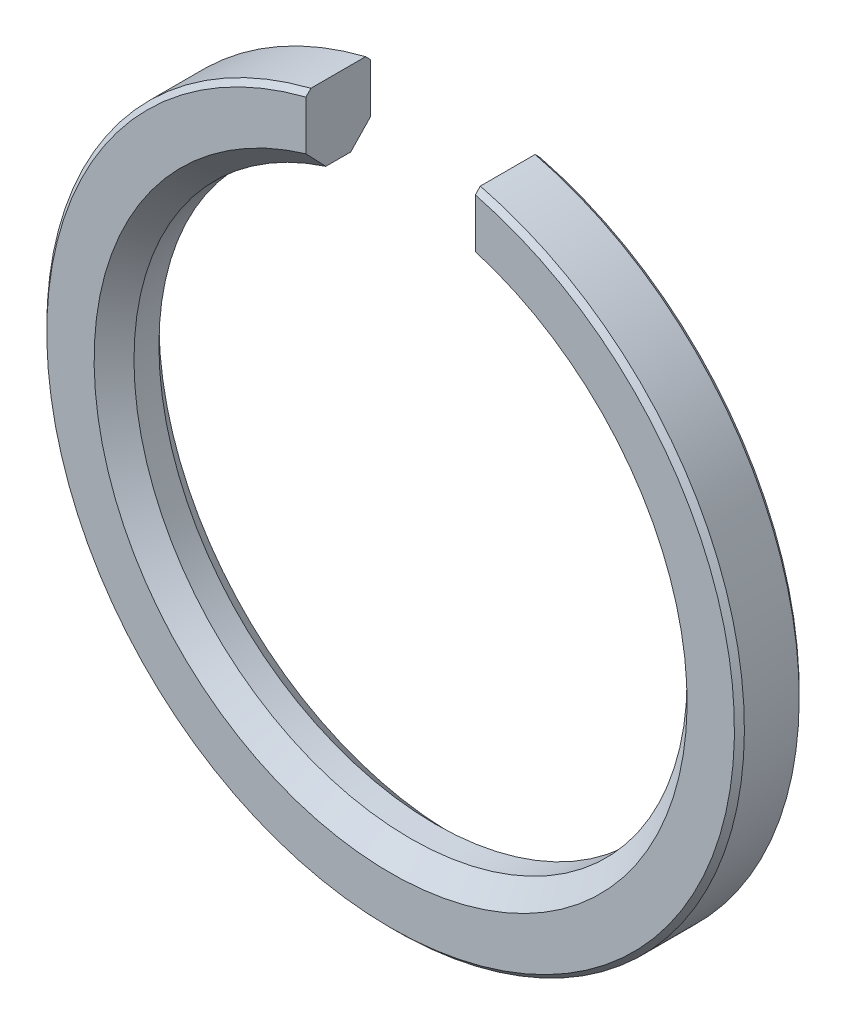
SolidWorks part; units mm, degrees
material "普通碳钢"
ref_plane "Front Plane" through (0, 0, 0) normal (0, 0, 1) x (1, 0, 0)
ref_plane "Top Plane" through (0, 0, 0) normal (0, 1, 0) x (1, 0, 0)
ref_plane "Right Plane" through (0, 0, 0) normal (1, 0, 0) x (0, 0, -1)
sketch "Sketch1" plane through (0, 0, 0) normal (0, 0, 1) x (1, 0, 0)
  circle A0 centre (0, 0) radius 27.75
  circle A1 centre (0, 0) radius 35
  dimension "D1" = 55.5
  dimension "D2" = 70
extrude "Boss-Extrude1" add sketch "Sketch1" along normal blind 6.5
sketch "Sketch2" plane through (0, 0, 6.5) normal (0, 0, 1) x (1, 0, 0)
  line L0 (0, 0) -> (8.5, 0)
  line L1 (8.5, 0) -> (8.5, 53.9047)
  line L2 (8.5, 53.9047) -> (-8.5, 53.9047)
  line L3 (-8.5, 53.9047) -> (-8.5, 0)
  line L4 (-8.5, 0) -> (0, 0)
  dimension "D1" = 8.5
  dimension "D2" = 8.5
extrude "Cut-Extrude1" cut sketch "Sketch2" against normal through all
chamfer "Chamfer1" distance 2 angle 45 2 edges at (0, -27.75, 0) (0, -27.75, 6.5)
chamfer "Chamfer2" distance 0.5 angle 45 2 edges at (0, -35, 0) (0, -35, 6.5)
